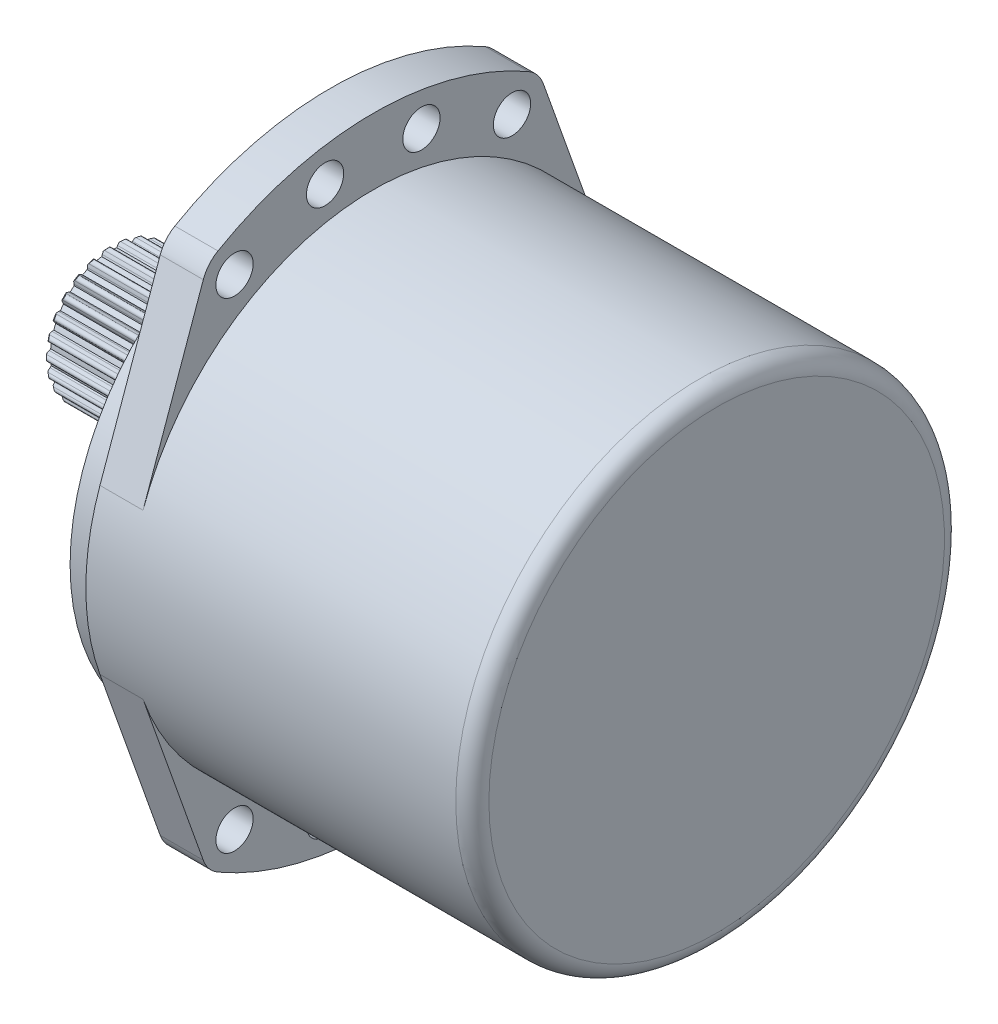
SolidWorks part; units mm, degrees
material "铸造合金钢"
ref_plane "Front Plane" through (0, 0, 0) normal (0, 0, 1) x (1, 0, 0)
ref_plane "Top Plane" through (0, 0, 0) normal (0, 1, 0) x (1, 0, 0)
ref_plane "Right Plane" through (0, 0, 0) normal (1, 0, 0) x (0, 0, -1)
sketch "Sketch1" plane through (0, 0, 0) normal (0, 0, 1) x (1, 0, 0)
  line L0 (-207.3, 187.5) -> (-207.3, 147.5)
  line L2 (-207.3, 147.5) -> (-10, 147.5)
  line L3 (0, 137.5) -> (0, 0)
  line L4 (-233.3, 187.5) -> (-233.3, 140)
  line L5 (-233.3, 140) -> (-250.3, 140)
  line L6 (-250.3, 140) -> (-250.3, 88)
  line L7 (-250.3, 88) -> (-280.8, 88)
  line L8 (-207.3, 187.5) -> (-233.3, 187.5)
  line L9 (-280.8, 88) -> (-280.8, 43)
  line L10 (-283.8, 35) -> (-366, 35)
  line L11 (-366, 35) -> (-366, 0)
  line L12 (-280.8, -35) -> (-366, -35) construction
  line L14 (-250.3, -88) -> (-280.8, -88) construction
  line L15 (-233.3, -140) -> (-250.3, -140) construction
  line L16 (-366, 0) -> (0, 0)
  line L17 (-207.3, -147.5) -> (0, -147.5) construction
  line L18 (-280.8, 43) -> (-283.8, 43)
  line L19 (-112.3393, 0) -> (70.717, 0) construction
  line L20 (-283.8, 43) -> (-283.8, 35)
  line L31 (-207.3, -187.5) -> (-233.3, -187.5) construction
  arc A0 (0, 137.5) -> (-10, 147.5) centre (-10, 137.5) ccw
  point P23 (0, 147.5)
  dimension "D9" = 70
  dimension "D11" = 10
  dimension "D1" = 26
  dimension "D2" = 233.3
  dimension "D3" = 17
  dimension "D4" = 47.5
  dimension "D5" = 366
  dimension "D6" = 176
  dimension "D7" = 280
  dimension "D8" = 295
  dimension "D10" = 375
  dimension "D13" = 8
  dimension "D12" = 3
revolve "Revolve1" add sketch "Sketch1" angle 360 about L19
sketch "Sketch2" plane through (-233.3, 0, 0) normal (-1, 0, 0) x (0, 0, 1)
  line L0 (0, 0) -> (-83.75, 145.0593) construction
  line L1 (0, -55) -> (0, 55) construction
  line L2 (-102.5947, 151.7583) -> (-138.9797, 49.4053)
  line L3 (0, 187.5) -> (0, -257.5942) construction
  line L4 (-283.8914, 0) -> (291.8442, 0) construction
  line L5 (55, 0) -> (-55, 0) construction
  line L6 (102.5947, 151.7583) -> (138.9797, 49.4053)
  line L7 (102.5947, -151.7583) -> (138.9797, -49.4053)
  line L8 (-102.5947, -151.7583) -> (-138.9797, -49.4053)
  line L9 (0, 0) -> (-29.0861, 164.9553) construction
  arc A1 (93.75, -162.3798) -> (93.75, 162.3798) centre (0, 0) ccw
  arc A2 (-138.9797, 49.4053) -> (-138.9797, -49.4053) centre (0, 0) ccw
  circle A3 centre (0, 0) radius 167.5 construction
  arc A4 (-93.75, 162.3798) -> (-102.5947, 151.7583) centre (-83.75, 145.0593) ccw
  arc A5 (93.75, 162.3798) -> (102.5947, 151.7583) centre (83.75, 145.0593) cw
  arc A6 (93.75, -162.3798) -> (102.5947, -151.7583) centre (83.75, -145.0593) ccw
  arc A7 (-93.75, -162.3798) -> (-102.5947, -151.7583) centre (-83.75, -145.0593) cw
  arc A8 (138.9797, -49.4053) -> (138.9797, 49.4053) centre (0, 0) ccw
  arc A9 (-93.75, 162.3798) -> (-93.75, -162.3798) centre (0, 0) ccw
  circle A10 centre (-83.75, 145.0593) radius 11.25
  circle A11 centre (-29.0861, 164.9553) radius 11.25
  circle A12 centre (29.0861, 164.9553) radius 11.25
  circle A13 centre (83.75, 145.0593) radius 11.25
  circle A14 centre (83.75, -145.0593) radius 11.25
  circle A15 centre (29.0861, -164.9553) radius 11.25
  circle A16 centre (-29.0861, -164.9553) radius 11.25
  circle A17 centre (-83.75, -145.0593) radius 11.25
  dimension "D1" = 295
  dimension "D2" = 335
  dimension "D4" = 22.5
  dimension "D6" = 20
  dimension "D3" = 30
  dimension "D5" = 20
extrude "Cut-Extrude1" cut sketch "Sketch2" against normal up to next
sketch "Sketch5" plane through (-366, 0, 0) normal (-1, 0, 0) x (0, 0, 1)
  arc A150 (37.2018, -11.1958) -> (37.9938, -8.1112) centre (37.0791, -9.5203) ccw
  arc A151 (37.9938, -8.1112) -> (36.4401, -6.6948) centre (24.1571, -21.7297) ccw
  arc A152 (36.4401, -6.6948) -> (35.6355, -6.0776) centre (25.7101, -19.8496) ccw
  arc A153 (35.6355, -6.0776) -> (36.0273, -2.9755) centre (0, 0) ccw
  arc A154 (36.0273, -2.9755) -> (36.9602, -2.5778) centre (29.8388, 12.8321) ccw
  arc A155 (36.9602, -2.5778) -> (38.8174, -1.5923) centre (28.8021, 15.0394) ccw
  arc A156 (38.8174, -1.5923) -> (38.8174, 1.5923) centre (38.2818, 0) ccw
  arc A157 (38.8174, 1.5923) -> (36.9602, 2.5778) centre (28.8021, -15.0394) ccw
  arc A158 (36.9602, 2.5778) -> (36.0273, 2.9755) centre (29.8388, -12.8321) ccw
  arc A159 (36.0273, 2.9755) -> (35.6355, 6.0776) centre (0, 0) ccw
  arc A160 (35.6355, 6.0776) -> (36.4401, 6.6948) centre (25.7101, 19.8496) ccw
  arc A161 (36.4401, 6.6948) -> (37.9938, 8.1112) centre (24.1571, 21.7297) ccw
  arc A162 (37.9938, 8.1112) -> (37.2018, 11.1958) centre (37.0791, 9.5203) ccw
  arc A163 (37.2018, 11.1958) -> (35.158, 11.6884) centre (31.6374, -7.4041) ccw
  arc A164 (35.158, 11.6884) -> (34.1555, 11.8417) centre (32.0926, -5.0084) ccw
  arc A165 (34.1555, 11.8417) -> (33.0045, 14.7488) centre (0, 0) ccw
  arc A166 (33.0045, 14.7488) -> (33.6303, 15.5468) centre (19.966, 25.6198) ccw
  arc A167 (33.6303, 15.5468) -> (34.783, 17.305) centre (17.9942, 27.0547) ccw
  arc A168 (34.783, 17.305) -> (33.2488, 20.0958) centre (33.5466, 18.4424) ccw
  arc A169 (33.2488, 20.0958) -> (31.1466, 20.0647) centre (32.4848, 0.6964) ccw
  arc A170 (31.1466, 20.0647) -> (30.1375, 19.9638) centre (32.3298, 3.1301) ccw
  arc A171 (30.1375, 19.9638) -> (28.2997, 22.4933) centre (0, 0) ccw
  arc A172 (28.2997, 22.4933) -> (28.7075, 23.4219) centre (12.9673, 29.7803) ccw
  arc A173 (28.7075, 23.4219) -> (29.3867, 25.4115) centre (10.7006, 30.6797) ccw
  arc A174 (29.3867, 25.4115) -> (27.2066, 27.7331) centre (27.9062, 26.2057) ccw
  arc A175 (27.2066, 27.7331) -> (25.1782, 27.1801) centre (31.291, 8.7531) ccw
  arc A176 (25.1782, 27.1801) -> (24.2259, 26.8315) centre (30.5357, 11.0718) ccw
  arc A177 (24.2259, 26.8315) -> (21.8167, 28.8245) centre (0, 0) ccw
  arc A178 (21.8167, 28.8245) -> (21.9808, 29.8253) centre (5.1539, 32.0695) ccw
  arc A179 (21.9808, 29.8253) -> (22.1438, 31.9214) centre (2.7347, 32.377) ccw
  arc A180 (22.1438, 31.9214) -> (19.4549, 33.6278) centre (20.5124, 32.3224) ccw
  arc A181 (19.4549, 33.6278) -> (17.6278, 32.5878) centre (28.1312, 16.2599) ccw
  arc A182 (17.6278, 32.5878) -> (16.7921, 32.0133) centre (26.8229, 18.3179) ccw
  arc A183 (16.7921, 32.0133) -> (13.963, 33.3445) centre (0, 0) ccw
  arc A184 (13.963, 33.3445) -> (13.873, 34.3547) centre (-2.9834, 32.3437) ccw
  arc A185 (13.873, 34.3547) -> (13.5096, 36.4254) centre (-5.403, 32.0399) ccw
  arc A186 (13.5096, 36.4254) -> (10.4808, 37.4096) centre (11.8297, 36.4081) ccw
  arc A187 (10.4808, 37.4096) -> (8.9697, 35.9478) centre (23.2037, 22.745) ccw
  arc A188 (8.9697, 35.9478) -> (8.3032, 35.1835) centre (21.4248, 24.413) ccw
  arc A189 (8.3032, 35.1835) -> (5.2318, 35.7694) centre (0, 0) ccw
  arc A190 (5.2318, 35.7694) -> (4.8935, 36.7254) centre (-10.9332, 30.5856) ccw
  arc A191 (4.8935, 36.7254) -> (4.0266, 38.6408) centre (-13.2012, 29.6896) ccw
  arc A192 (4.0266, 38.6408) -> (0.8482, 38.8407) centre (2.4037, 38.2063) ccw
  arc A193 (0.8482, 38.8407) -> (-0.252, 37.0491) centre (16.8182, 27.801) ccw
  arc A194 (-0.252, 37.0491) -> (-0.7075, 36.1431) centre (14.6804, 28.9742) ccw
  arc A195 (-0.7075, 36.1431) -> (-3.828, 35.9467) centre (0, 0) ccw
  arc A196 (-3.828, 35.9467) -> (-4.3935, 36.7886) centre (-18.1961, 26.9057) ccw
  arc A197 (-4.3935, 36.7886) -> (-5.7095, 38.4282) centre (-20.17, 25.4738) ccw
  arc A198 (-5.7095, 38.4282) -> (-8.8378, 37.8314) centre (-7.1733, 37.6037) ccw
  arc A199 (-8.8378, 37.8314) -> (-9.4578, 35.8225) centre (9.3761, 31.1101) ccw
  arc A200 (-9.4578, 35.8225) -> (-9.6737, 34.8316) centre (7.0136, 31.7147) ccw
  arc A201 (-9.6737, 34.8316) -> (-12.6473, 33.8654) centre (0, 0) ccw
  arc A202 (-12.6473, 33.8654) -> (-13.4044, 34.5402) centre (-24.3156, 21.5353) ccw
  arc A203 (-13.4044, 34.5402) -> (-15.0868, 35.801) centre (-25.8714, 19.6575) ccw
  arc A204 (-15.0868, 35.801) -> (-17.9684, 34.445) centre (-16.2996, 34.6384) ccw
  arc A205 (-17.9684, 34.445) -> (-18.0693, 32.345) centre (1.3447, 32.4644) ccw
  arc A206 (-18.0693, 32.345) -> (-18.032, 31.3316) centre (-1.0939, 32.4626) ccw
  arc A207 (-18.032, 31.3316) -> (-20.672, 29.6562) centre (0, 0) ccw
  arc A208 (-20.672, 29.6562) -> (-21.5731, 30.1215) centre (-28.9073, 14.8117) ccw
  arc A209 (-21.5731, 30.1215) -> (-23.5162, 30.9243) centre (-29.9472, 12.6059) ccw
  arc A210 (-23.5162, 30.9243) -> (-25.97, 28.8943) centre (-24.4017, 29.4966) ccw
  arc A211 (-25.97, 28.8943) -> (-25.5455, 26.8352) centre (-6.7711, 31.7789) ccw
  arc A212 (-25.5455, 26.8352) -> (-25.2574, 25.8629) centre (-9.1326, 31.1707) ccw
  arc A213 (-25.2574, 25.8629) -> (-27.3977, 23.5836) centre (0, 0) ccw
  arc A214 (-27.3977, 23.5836) -> (-28.3863, 23.8101) centre (-31.6826, 7.1574) ccw
  arc A215 (-28.3863, 23.8101) -> (-30.4679, 24.1045) centre (-32.1414, 4.7623) ccw
  arc A216 (-30.4679, 24.1045) -> (-32.3399, 21.528) centre (-30.9706, 22.5015) ccw
  arc A217 (-32.3399, 21.528) -> (-31.4166, 19.6392) centre (-14.4615, 29.0966) ccw
  arc A218 (-31.4166, 19.6392) -> (-30.8957, 18.7691) centre (-16.5975, 27.9202) ccw
  arc A219 (-30.8957, 18.7691) -> (-32.402, 16.0291) centre (0, 0) ccw
  arc A220 (-32.402, 16.0291) -> (-33.4158, 16.0027) centre (-32.4672, -0.9466) ccw
  arc A221 (-33.4158, 16.0027) -> (-35.5053, 15.7701) centre (-32.3159, -3.3805) ccw
  arc A222 (-35.5053, 15.7701) -> (-36.6776, 12.8091) centre (-35.5935, 14.0925) ccw
  arc A223 (-36.6776, 12.8091) -> (-35.3137, 11.2092) centre (-21.2432, 24.5861) ccw
  arc A224 (-35.3137, 11.2092) -> (-34.5927, 10.496) centre (-23.0196, 22.9154) ccw
  arc A225 (-34.5927, 10.496) -> (-35.3703, 7.4675) centre (0, 0) ccw
  arc A226 (-35.3703, 7.4675) -> (-36.3457, 7.1898) centre (-31.2118, -8.9911) ccw
  arc A227 (-36.3457, 7.1898) -> (-38.3117, 6.4449) centre (-30.4599, -11.311) ccw
  arc A228 (-38.3117, 6.4449) -> (-38.7108, 3.2853) centre (-37.9799, 4.798) ccw
  arc A229 (-38.7108, 3.2853) -> (-36.9919, 2.0749) centre (-26.6901, 18.5307) ccw
  arc A230 (-36.9919, 2.0749) -> (-36.1162, 1.5633) centre (-27.9952, 16.4707) ccw
  arc A231 (-36.1162, 1.5633) -> (-36.1162, -1.5633) centre (0, 0) ccw
  arc A232 (-36.1162, -1.5633) -> (-36.9919, -2.0749) centre (-27.9952, -16.4707) ccw
  arc A233 (-36.9919, -2.0749) -> (-38.7108, -3.2853) centre (-26.6901, -18.5307) ccw
  arc A234 (-38.7108, -3.2853) -> (-38.3117, -6.4449) centre (-37.9799, -4.798) ccw
  arc A235 (-38.3117, -6.4449) -> (-36.3457, -7.1898) centre (-30.4599, 11.311) ccw
  arc A236 (-36.3457, -7.1898) -> (-35.3703, -7.4675) centre (-31.2118, 8.9911) ccw
  arc A237 (-35.3703, -7.4675) -> (-34.5927, -10.496) centre (0, 0) ccw
  arc A238 (-34.5927, -10.496) -> (-35.3137, -11.2092) centre (-23.0196, -22.9154) ccw
  arc A239 (-35.3137, -11.2092) -> (-36.6776, -12.8091) centre (-21.2432, -24.5861) ccw
  arc A240 (-36.6776, -12.8091) -> (-35.5053, -15.7701) centre (-35.5935, -14.0925) ccw
  arc A241 (-35.5053, -15.7701) -> (-33.4158, -16.0027) centre (-32.3159, 3.3805) ccw
  arc A242 (-33.4158, -16.0027) -> (-32.402, -16.0291) centre (-32.4672, 0.9466) ccw
  arc A243 (-32.402, -16.0291) -> (-30.8957, -18.7691) centre (0, 0) ccw
  arc A244 (-30.8957, -18.7691) -> (-31.4166, -19.6392) centre (-16.5975, -27.9202) ccw
  arc A245 (-31.4166, -19.6392) -> (-32.3399, -21.528) centre (-14.4615, -29.0966) ccw
  arc A246 (-32.3399, -21.528) -> (-30.4679, -24.1045) centre (-30.9706, -22.5015) ccw
  arc A247 (-30.4679, -24.1045) -> (-28.3863, -23.8101) centre (-32.1414, -4.7623) ccw
  arc A248 (-28.3863, -23.8101) -> (-27.3977, -23.5836) centre (-31.6826, -7.1574) ccw
  arc A249 (-27.3977, -23.5836) -> (-25.2574, -25.8629) centre (0, 0) ccw
  arc A250 (-25.2574, -25.8629) -> (-25.5455, -26.8352) centre (-9.1326, -31.1707) ccw
  arc A251 (-25.5455, -26.8352) -> (-25.97, -28.8943) centre (-6.7711, -31.7789) ccw
  arc A252 (-25.97, -28.8943) -> (-23.5162, -30.9243) centre (-24.4017, -29.4966) ccw
  arc A253 (-23.5162, -30.9243) -> (-21.5731, -30.1215) centre (-29.9472, -12.6059) ccw
  arc A254 (-21.5731, -30.1215) -> (-20.672, -29.6562) centre (-28.9073, -14.8117) ccw
  arc A255 (-20.672, -29.6562) -> (-18.032, -31.3316) centre (0, 0) ccw
  arc A256 (-18.032, -31.3316) -> (-18.0693, -32.345) centre (-1.0939, -32.4626) ccw
  arc A257 (-18.0693, -32.345) -> (-17.9684, -34.445) centre (1.3447, -32.4644) ccw
  arc A258 (-17.9684, -34.445) -> (-15.0868, -35.801) centre (-16.2996, -34.6384) ccw
  arc A259 (-15.0868, -35.801) -> (-13.4044, -34.5402) centre (-25.8714, -19.6575) ccw
  arc A260 (-13.4044, -34.5402) -> (-12.6473, -33.8654) centre (-24.3156, -21.5353) ccw
  arc A261 (-12.6473, -33.8654) -> (-9.6737, -34.8316) centre (0, 0) ccw
  arc A262 (-9.6737, -34.8316) -> (-9.4578, -35.8225) centre (7.0136, -31.7147) ccw
  arc A263 (-9.4578, -35.8225) -> (-8.8378, -37.8314) centre (9.3761, -31.1101) ccw
  arc A264 (-8.8378, -37.8314) -> (-5.7095, -38.4282) centre (-7.1733, -37.6037) ccw
  arc A265 (-5.7095, -38.4282) -> (-4.3935, -36.7886) centre (-20.17, -25.4738) ccw
  arc A266 (-4.3935, -36.7886) -> (-3.828, -35.9467) centre (-18.1961, -26.9057) ccw
  arc A267 (-3.828, -35.9467) -> (-0.7075, -36.1431) centre (0, 0) ccw
  arc A268 (-0.7075, -36.1431) -> (-0.252, -37.0491) centre (14.6804, -28.9742) ccw
  arc A269 (-0.252, -37.0491) -> (0.8482, -38.8407) centre (16.8182, -27.801) ccw
  arc A270 (0.8482, -38.8407) -> (4.0266, -38.6408) centre (2.4037, -38.2063) ccw
  arc A271 (4.0266, -38.6408) -> (4.8935, -36.7254) centre (-13.2012, -29.6896) ccw
  arc A272 (4.8935, -36.7254) -> (5.2318, -35.7694) centre (-10.9332, -30.5856) ccw
  arc A273 (5.2318, -35.7694) -> (8.3032, -35.1835) centre (0, 0) ccw
  arc A274 (8.3032, -35.1835) -> (8.9697, -35.9478) centre (21.4248, -24.413) ccw
  arc A275 (8.9697, -35.9478) -> (10.4808, -37.4096) centre (23.2037, -22.745) ccw
  arc A276 (10.4808, -37.4096) -> (13.5096, -36.4254) centre (11.8297, -36.4081) ccw
  arc A277 (13.5096, -36.4254) -> (13.873, -34.3547) centre (-5.403, -32.0399) ccw
  arc A278 (13.873, -34.3547) -> (13.963, -33.3445) centre (-2.9834, -32.3437) ccw
  arc A279 (13.963, -33.3445) -> (16.7921, -32.0133) centre (0, 0) ccw
  arc A280 (16.7921, -32.0133) -> (17.6278, -32.5878) centre (26.8229, -18.3179) ccw
  arc A281 (17.6278, -32.5878) -> (19.4549, -33.6278) centre (28.1312, -16.2599) ccw
  arc A282 (19.4549, -33.6278) -> (22.1438, -31.9214) centre (20.5124, -32.3224) ccw
  arc A283 (22.1438, -31.9214) -> (21.9808, -29.8253) centre (2.7347, -32.377) ccw
  arc A284 (21.9808, -29.8253) -> (21.8167, -28.8245) centre (5.1539, -32.0695) ccw
  arc A285 (21.8167, -28.8245) -> (24.2259, -26.8315) centre (0, 0) ccw
  arc A286 (24.2259, -26.8315) -> (25.1782, -27.1801) centre (30.5357, -11.0718) ccw
  arc A287 (25.1782, -27.1801) -> (27.2066, -27.7331) centre (31.291, -8.7531) ccw
  arc A288 (27.2066, -27.7331) -> (29.3867, -25.4115) centre (27.9062, -26.2057) ccw
  arc A289 (29.3867, -25.4115) -> (28.7075, -23.4219) centre (10.7006, -30.6797) ccw
  arc A290 (28.7075, -23.4219) -> (28.2997, -22.4933) centre (12.9673, -29.7803) ccw
  arc A291 (28.2997, -22.4933) -> (30.1375, -19.9638) centre (0, 0) ccw
  arc A292 (30.1375, -19.9638) -> (31.1466, -20.0647) centre (32.3298, -3.1301) ccw
  arc A293 (31.1466, -20.0647) -> (33.2488, -20.0958) centre (32.4848, -0.6964) ccw
  arc A294 (33.2488, -20.0958) -> (34.783, -17.305) centre (33.5466, -18.4424) ccw
  arc A295 (34.783, -17.305) -> (33.6303, -15.5468) centre (17.9942, -27.0547) ccw
  arc A296 (33.6303, -15.5468) -> (33.0045, -14.7488) centre (19.966, -25.6198) ccw
  arc A297 (33.0045, -14.7488) -> (34.1555, -11.8417) centre (0, 0) ccw
  arc A298 (34.1555, -11.8417) -> (35.158, -11.6884) centre (32.0926, 5.0084) ccw
  arc A299 (35.158, -11.6884) -> (37.2018, -11.1958) centre (31.6374, 7.4041) ccw
extrude "Boss-Extrude1" add sketch "Sketch5" against normal up to next
sketch "Sketch7" plane through (0, 0, 0) normal (0, 1, 0) x (1, 0, 0)
  line L0 (-366.384, 40.044) -> (-364.384, 40.044)
  line L1 (-364.384, 40.044) -> (-366.384, 38.044)
  line L2 (-366.384, 38.044) -> (-366.384, 40.044)
  line L3 (-366, 39.6599) -> (-366.384, 40.044) construction
  dimension "D1" = 45
  dimension "D2" = 2
  dimension "D3" = 90
revolve "Cut-Revolve1" cut sketch "Sketch7" angle 360 about axis through (-112.3393, 0, 0) along (-1, 0, 0)
